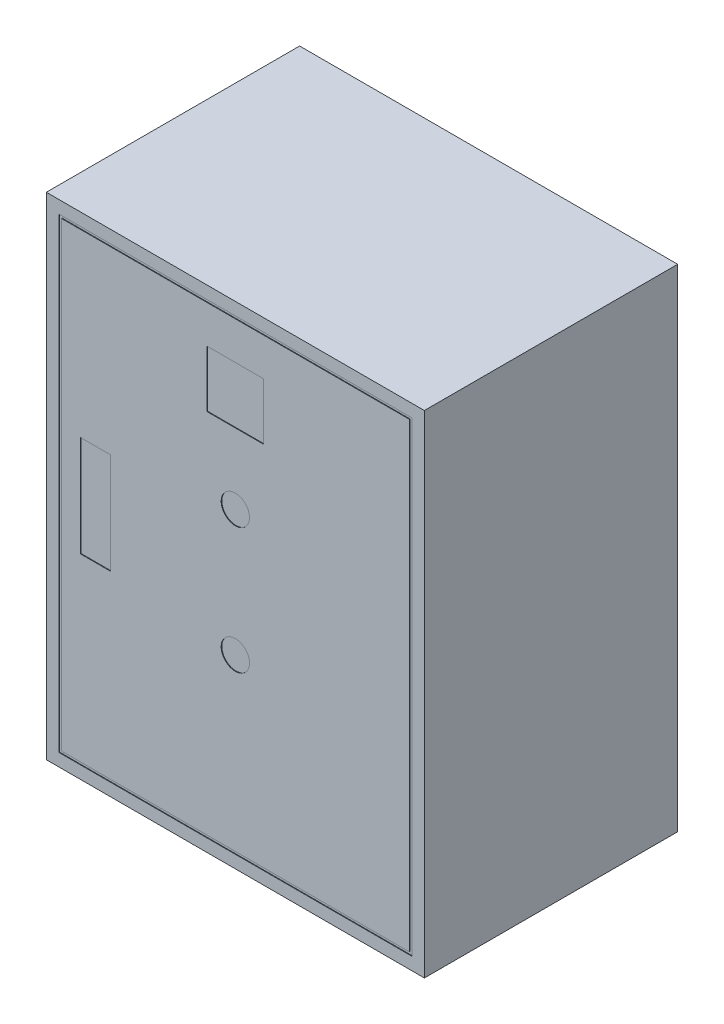
from build123d import *

# Parameters (mm, degrees)
SKETCH1_W           = 300
SKETCH1_H           = 390
BOSS_EXTRUDE1_DEPTH = 200
SHELL1_T            = -1.5
SKETCH2_W           = 300
SKETCH2_H           = 390
BOSS_EXTRUDE2_DEPTH = 1
SKETCH3_W           = 280
SKETCH3_H           = 370
SKETCH3_W_2         = 276
SKETCH3_H_2         = 366
SKETCH3_R           = 11.25
SKETCH3_W_3         = 24
SKETCH3_H_3         = 80
SKETCH3_W_4         = 45
SKETCH3_H_4         = 45
CUT_EXTRUDE1_DEPTH  = 0.5


with BuildPart() as part:
    # Sketch1 → Boss-Extrude1 (new body)
    with BuildSketch(Plane.XY):
        with Locations((150, 195)):
            Rectangle(SKETCH1_W, SKETCH1_H)
    extrude(amount=BOSS_EXTRUDE1_DEPTH)

    # Shell1
    shell1_openings = [part.faces().sort_by_distance(p)[0] for p in [
        (150, 195, 200),
    ]]
    offset(amount=SHELL1_T, openings=shell1_openings, kind=Kind.INTERSECTION)

    # Sketch2 → Boss-Extrude2 (add)
    with BuildSketch(Plane.XY.offset(200)):
        with Locations((150, 195)):
            Rectangle(SKETCH2_W, SKETCH2_H)
    extrude(amount=BOSS_EXTRUDE2_DEPTH)

    # Sketch3 → Cut-Extrude1 (cut)
    # profile 1 of 5: a face of its own
    with BuildSketch(Plane.XY.offset(201)):
        with Locations((150, 195)):
            Rectangle(SKETCH3_W, SKETCH3_H)
        with Locations((150, 195)):
            Rectangle(SKETCH3_W_2, SKETCH3_H_2, mode=Mode.SUBTRACT)
    # profile 2 of 5: a face of its own
    with BuildSketch(Plane.XY.offset(201)):
        with Locations((150, 247)):
            Circle(SKETCH3_R)
    # profile 3 of 5: a face of its own
    with BuildSketch(Plane.XY.offset(201)):
        with Locations((150, 147)):
            Circle(SKETCH3_R)
    # profile 4 of 5: a face of its own
    with BuildSketch(Plane.XY.offset(201)):
        with Locations((39, 195)):
            Rectangle(SKETCH3_W_3, SKETCH3_H_3)
    # profile 5 of 5: a face of its own
    with BuildSketch(Plane.XY.offset(201)):
        with Locations((150, 325.5)):
            Rectangle(SKETCH3_W_4, SKETCH3_H_4)
    extrude(amount=-CUT_EXTRUDE1_DEPTH, mode=Mode.SUBTRACT)


solid = part.part
